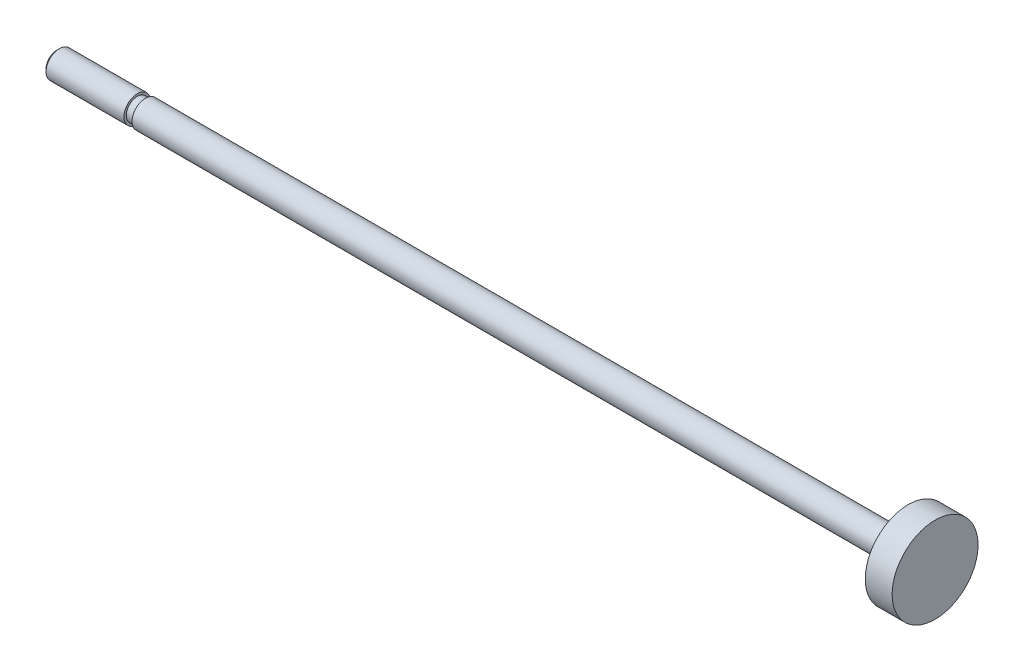
from build123d import *


with BuildPart() as part:
    # Sketch1 → Revolve1 (revolve)
    with BuildSketch(Plane(origin=(0, 0, 0), x_dir=(-1, 0, 0), z_dir=(0, 0, -1)), mode=Mode.PRIVATE) as revolve1_sk:
        Polygon((-135.5, 8), (-135.5, 0), (28, 0), (28, 2.0095), (27.5095, 2.5), (13, 2.5), (13, 2.065), (11.5, 2.065), (11.5, 2.5), (-130.5, 2.5), (-130.5, 8), align=None)
    revolve(revolve1_sk.sketch.rotate(Axis((135.5, 0, 0), (-1, 0, 0)), 270), axis=Axis((135.5, 0, 0), (-1, 0, 0)))


solid = part.part
